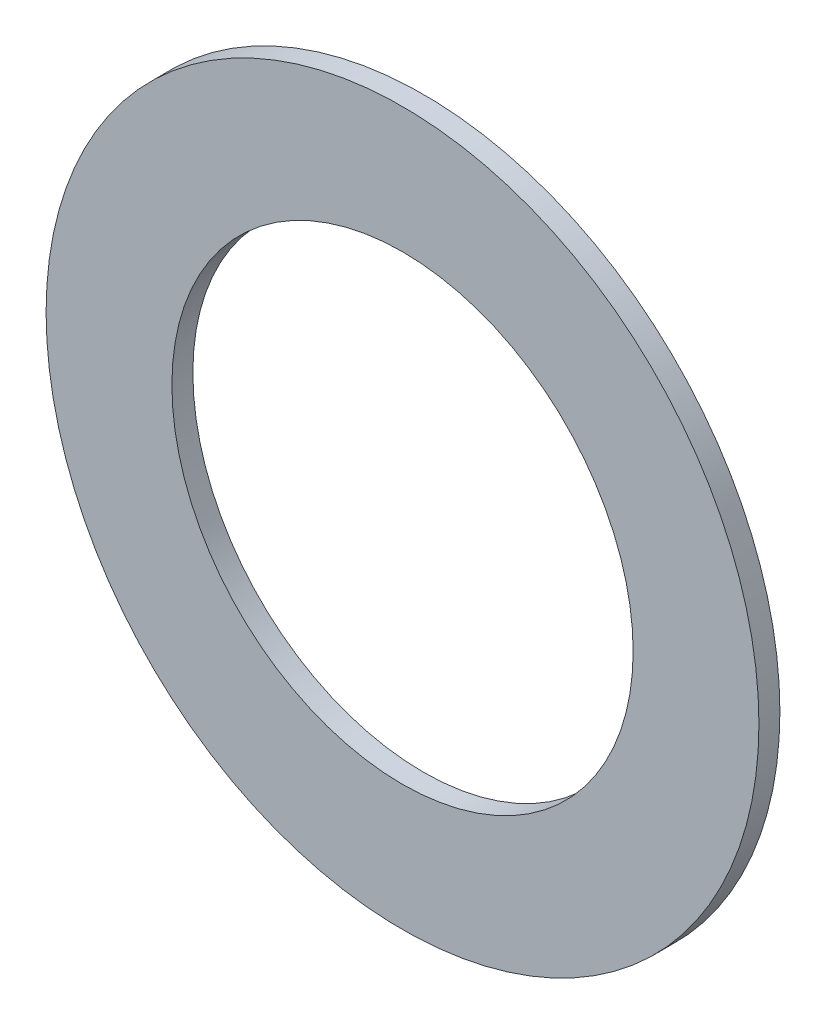
from build123d import *

# Parameters (mm, degrees)
SKETCH1_R           = 8.5
SKETCH1_R_2         = 5.5
BOSS_EXTRUDE1_DEPTH = 0.5


with BuildPart() as part:
    # Sketch1 → Boss-Extrude1 (new body)
    with BuildSketch(Plane.XY):
        Circle(SKETCH1_R)
        Circle(SKETCH1_R_2, mode=Mode.SUBTRACT)
    extrude(amount=BOSS_EXTRUDE1_DEPTH)


solid = part.part
